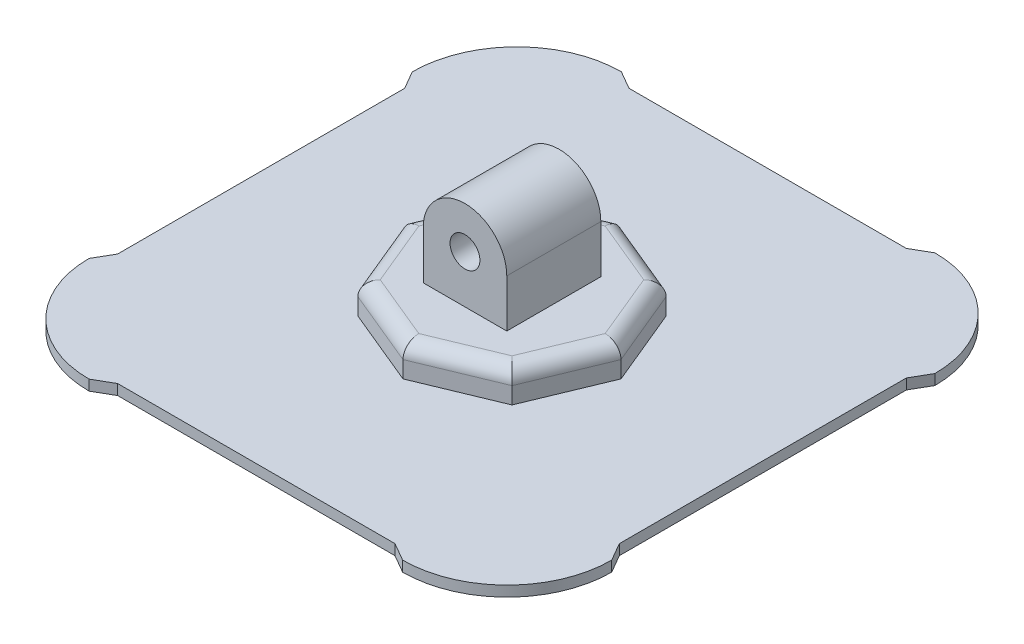
from build123d import *

# Parameters (mm, degrees)
BOSS_EXTRUDE1_DEPTH = 1
BOSS_EXTRUDE2_DEPTH = 3
FILLET1_R           = 1.4
SKETCH3_R           = 1.426316434
BOSS_EXTRUDE3_DEPTH = 4.5


with BuildPart() as part:
    # Sketch1 → Boss-Extrude1 (new body)
    with BuildSketch(Plane(origin=(0, 0, 0), x_dir=(1, 0, 0), z_dir=(0, 1, 0))):
        with BuildLine():
            Line((-15, -25.462186482), (-13.267949192, -24.462186482))
            Line((-13.267949192, -24.462186482), (13.267949192, -24.462186482))
            Line((13.267949192, -24.462186482), (15, -25.462186482))
            ThreePointArc((15, -25.462186482), (22.071067812, -22.533254294), (25, -15.462186482))
            Line((25, -15.462186482), (24, -13.730135674))
            Line((24, -13.730135674), (24, 13.730135674))
            Line((24, 13.730135674), (25, 15.462186482))
            ThreePointArc((25, 15.462186482), (22.071067812, 22.533254294), (15, 25.462186482))
            Line((15, 25.462186482), (13.267949192, 24.462186482))
            Line((13.267949192, 24.462186482), (-13.267949192, 24.462186482))
            Line((-13.267949192, 24.462186482), (-15, 25.462186482))
            ThreePointArc((-15, 25.462186482), (-22.071067812, 22.533254294), (-25, 15.462186482))
            Line((-25, 15.462186482), (-24, 13.730135674))
            Line((-24, 13.730135674), (-24, -13.730135674))
            Line((-24, -13.730135674), (-25, -15.462186482))
            ThreePointArc((-25, -15.462186482), (-22.071067812, -22.533254294), (-15, -25.462186482))
        make_face()
    extrude(amount=BOSS_EXTRUDE1_DEPTH)

    # Sketch2 → Boss-Extrude2 (add)
    with BuildSketch(Plane(origin=(0, 1, 0), x_dir=(1, 0, 0), z_dir=(0, 1, 0))):
        Polygon((0, -10.429037626), (7.374443227, -7.374443227), (10.429037626, 0), (-10.429037626, 0), (-7.374443227, -7.374443227), align=None)
        Polygon((0, 10.429037626), (-7.374443227, 7.374443227), (-10.429037626, 0), (10.429037626, 0), (7.374443227, 7.374443227), align=None)
    extrude(amount=BOSS_EXTRUDE2_DEPTH)

    # Fillet1
    fillet1_edges = [part.edges().sort_by_distance(p)[0] for p in [
        (3.687221613, 4, 8.901740426),
        (8.901740426, 4, 3.687221613),
        (8.901740426, 4, -3.687221613),
        (3.687221613, 4, -8.901740426),
        (-3.687221613, 4, -8.901740426),
        (-8.901740426, 4, -3.687221613),
        (-8.901740426, 4, 3.687221613),
        (-3.687221613, 4, 8.901740426),
    ]]
    fillet(fillet1_edges, radius=FILLET1_R)

    # Sketch3 → Boss-Extrude3 (add, symmetric)
    with BuildSketch(Plane.XY):
        with BuildLine():
            ThreePointArc((4, 8.569064594), (0.167778924, 12.565544324), (-3.985925116, 8.904327129))
            Line((-3.985925116, 8.904327129), (-3.985925116, 4))
            Line((-3.985925116, 4), (4, 4))
            Line((4, 4), (4, 8.569064594))
        make_face()
        with Locations((0, 8.569064594)):
            Circle(SKETCH3_R, mode=Mode.SUBTRACT)
    extrude(amount=BOSS_EXTRUDE3_DEPTH, both=True)


solid = part.part
